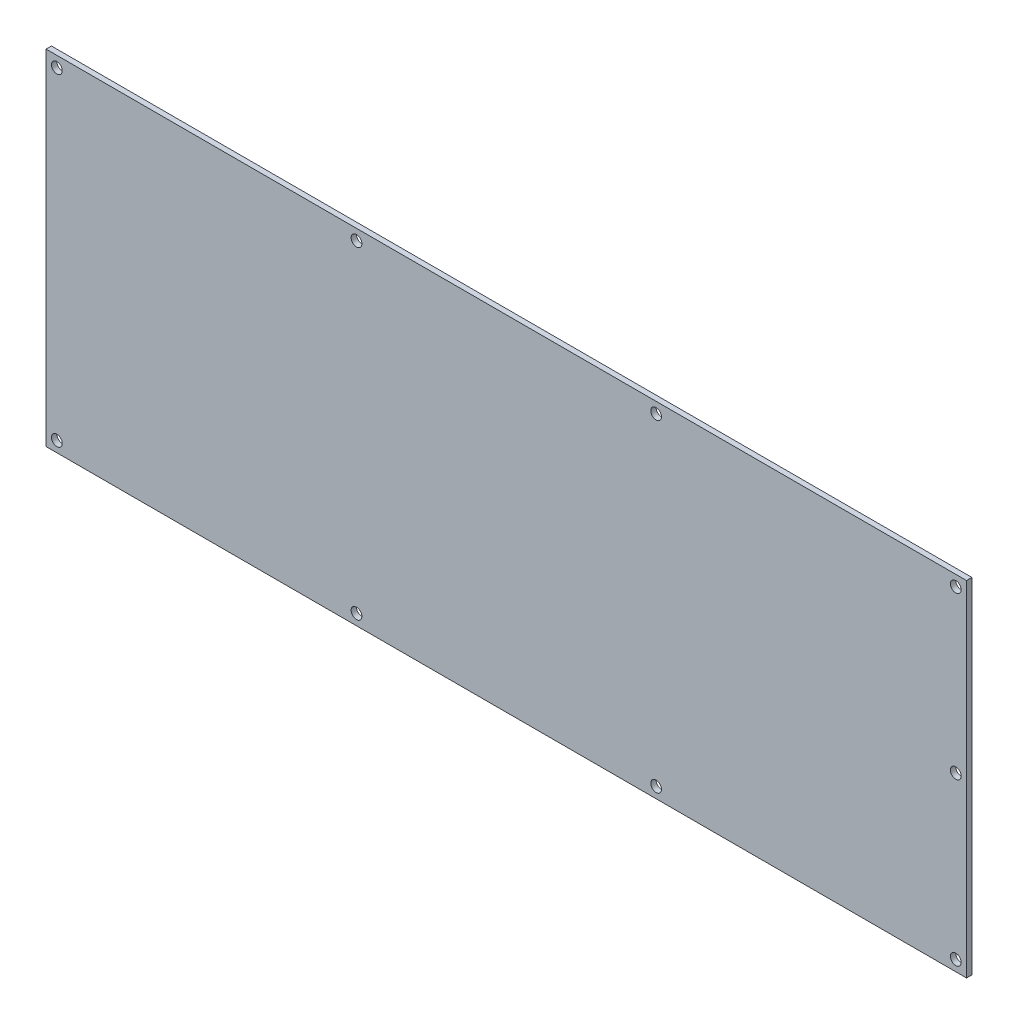
from build123d import *

# Parameters (mm, degrees)
SKETCH1_W           = 855.022462921
SKETCH1_H           = 319.761568038
SKETCH1_R           = 5
BOSS_EXTRUDE1_DEPTH = 5


with BuildPart() as part:
    # Sketch1 → Boss-Extrude1 (new body)
    with BuildSketch(Plane.XY):
        with Locations((427.511231461, 159.880784019)):
            Rectangle(SKETCH1_W, SKETCH1_H)
        with Locations((10, 309.761568038)):
            Circle(SKETCH1_R, mode=Mode.SUBTRACT)
        with Locations((845.022462921, 309.761568038)):
            Circle(SKETCH1_R, mode=Mode.SUBTRACT)
        with Locations((10, 10)):
            Circle(SKETCH1_R, mode=Mode.SUBTRACT)
        with Locations((845.022462921, 10)):
            Circle(SKETCH1_R, mode=Mode.SUBTRACT)
        with Locations((288.340820974, 309.761568038)):
            Circle(SKETCH1_R, mode=Mode.SUBTRACT)
        with Locations((288.340820974, 10)):
            Circle(SKETCH1_R, mode=Mode.SUBTRACT)
        with Locations((566.681641947, 309.761568038)):
            Circle(SKETCH1_R, mode=Mode.SUBTRACT)
        with Locations((566.681641947, 10)):
            Circle(SKETCH1_R, mode=Mode.SUBTRACT)
        with Locations((845.022462921, 159.880784019)):
            Circle(SKETCH1_R, mode=Mode.SUBTRACT)
    extrude(amount=BOSS_EXTRUDE1_DEPTH)


solid = part.part
